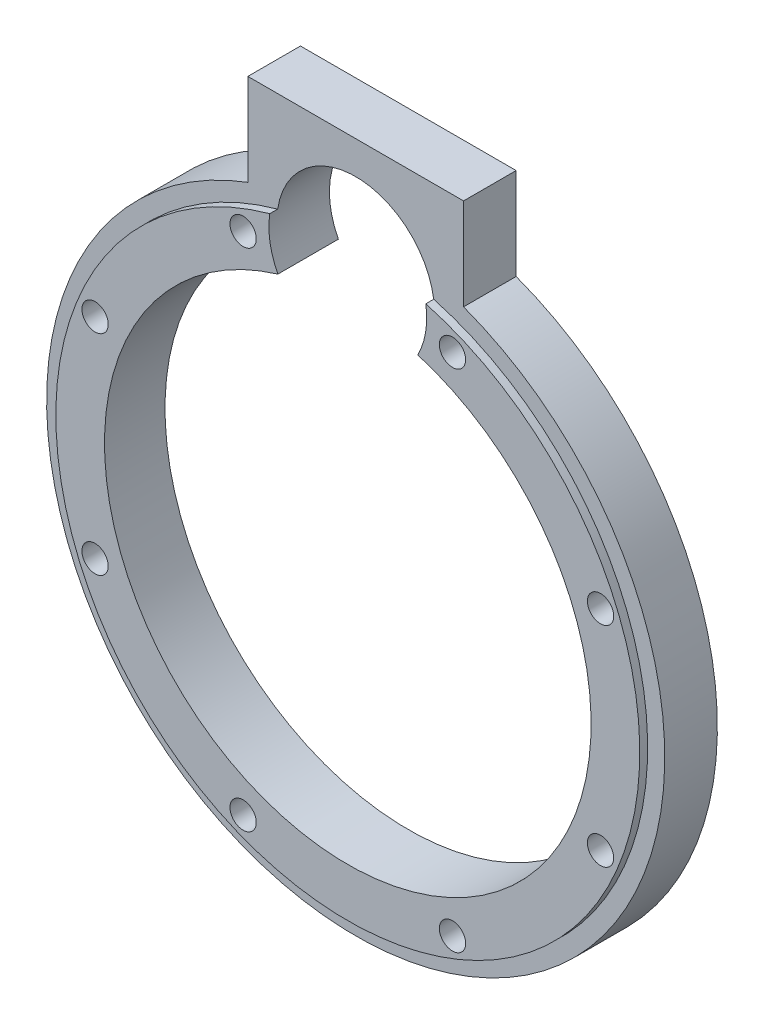
SolidWorks part; units mm, degrees
material "Q235A"
ref_plane "前视基准面" through (0, 0, 0) normal (0, 0, 1) x (1, 0, 0)
ref_plane "上视基准面" through (0, 0, 0) normal (0, 1, 0) x (1, 0, 0)
ref_plane "右视基准面" through (0, 0, 0) normal (1, 0, 0) x (0, 0, -1)
sketch "草图1" plane through (0, 0, 0) normal (0, 0, 1) x (1, 0, 0)
  circle A0 centre (0, 0) radius 117.5
  circle A1 centre (0, 0) radius 92.5
  dimension "D1" = 235
  dimension "D2" = 185
extrude "凸台-拉伸1" add sketch "草图1" along normal blind 20
sketch "草图2" plane through (0, 0, 20) normal (0, 0, 1) x (1, 0, 0)
  line L0 (0, 0) -> (0, 118.75) construction
  line L2 (-41, 92.5) -> (41, 92.5)
  line L3 (-41, 92.5) -> (-41, 145)
  line L4 (-41, 145) -> (41, 145)
  line L5 (41, 92.5) -> (41, 145)
  line L6 (-41, 92.5) -> (41, 145) construction
  line L7 (-41, 145) -> (41, 92.5) construction
  circle A1 centre (0, 0) radius 92.5 construction
  dimension "D1" = 82
  dimension "D2" = 145
extrude "凸台-拉伸2" add sketch "草图2" against normal through all
sketch "草图7" plane through (0, 0, 20) normal (0, 0, 1) x (1, 0, 0)
  circle A0 centre (0, 0) radius 92.5 construction
  circle A1 centre (0, 0) radius 92.5
  circle A2 centre (0, 0) radius 111
  dimension "D1" = 222
extrude "凸台-拉伸3" add sketch "草图7" along normal blind 3
sketch "草图3" plane through (0, 0, 0) normal (0, 0, -1) x (-1, 0, 0)
  circle A0 centre (0, 102.5) radius 30
  dimension "D1" = 60
extrude "切除-拉伸1" cut sketch "草图3" against normal through all
hole_wizard "M8 间隙孔1" positions "草图8" profile "草图9" hole size "M8" standard "ISO" end condition through all
sketch "草图8" plane through (0, 0, 0) normal (0, 0, -1) x (-1, 0, 0)
  point P0 (-39.7991, 96.0835)
  point P3 (-96.0835, 39.7991)
  point P6 (-96.0835, -39.7991)
  point P9 (-39.7991, -96.0835)
  point P12 (39.7991, -96.0835)
  point P15 (96.0835, -39.7991)
  point P18 (96.0835, 39.7991)
  point P21 (39.7991, 96.0835)
sketch "草图9" plane through (39.7991, 96.0835, 0) normal (1, 0, 0) x (0, 1, 0)
  line L0 (0, 0) -> (0, 23)
  line L1 (0, 23) -> (5, 23)
  line L2 (5, 23) -> (5, 0)
  line L5 (5, 0) -> (0, 0)
  line L11 (0, -6.35) -> (0, 107.95) construction
  dimension "通孔孔直径" = 10
  dimension "通孔孔深度" = 23
